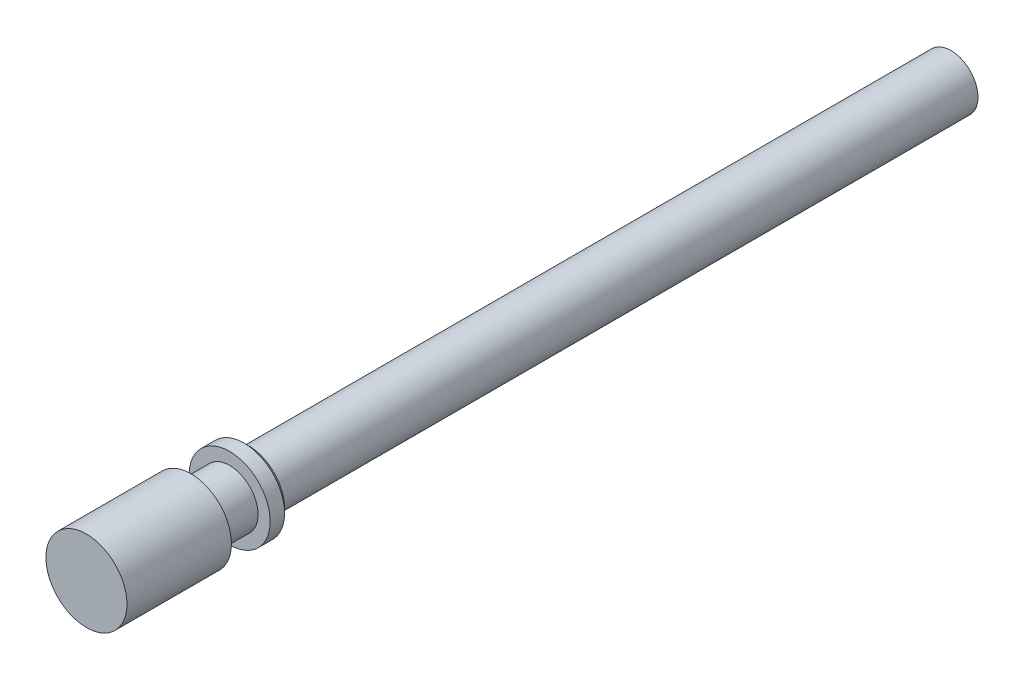
from build123d import *

# Parameters (mm, degrees)
SKETCH1_R           = 3
BOSS_EXTRUDE1_DEPTH = 96
SKETCH2_R           = 4.5
BOSS_EXTRUDE2_DEPTH = 18
CUT_EXTRUDE1_START  = -11.6
SKETCH3_OUTSIDE_W   = 30.368
SKETCH3_OUTSIDE_H   = 30.368
SKETCH3_OUTSIDE_R   = 3.15
CUT_EXTRUDE1_DEPTH  = 4.3
CHAMFER1_SIZE       = 0.5


with BuildPart() as part:
    # Sketch1 → Boss-Extrude1 (new body)
    with BuildSketch(Plane.XY):
        Circle(SKETCH1_R)
    extrude(amount=BOSS_EXTRUDE1_DEPTH)

    # Sketch2 → Boss-Extrude2 (add)
    with BuildSketch(Plane.XY.offset(96)):
        Circle(SKETCH2_R)
    extrude(amount=-BOSS_EXTRUDE2_DEPTH)

    # Sketch3 outside → Cut-Extrude1 (cut)
    with BuildSketch(Plane.XY.offset(96).offset(CUT_EXTRUDE1_START)):
        Rectangle(SKETCH3_OUTSIDE_W, SKETCH3_OUTSIDE_H)
        Circle(SKETCH3_OUTSIDE_R, mode=Mode.SUBTRACT)
    extrude(amount=-CUT_EXTRUDE1_DEPTH, mode=Mode.SUBTRACT)

    # Chamfer1
    chamfer1_edges = [part.edges().sort_by_distance(p)[0] for p in [
        (-4.5, 0, 78),
    ]]
    chamfer(chamfer1_edges, length=CHAMFER1_SIZE)


solid = part.part
